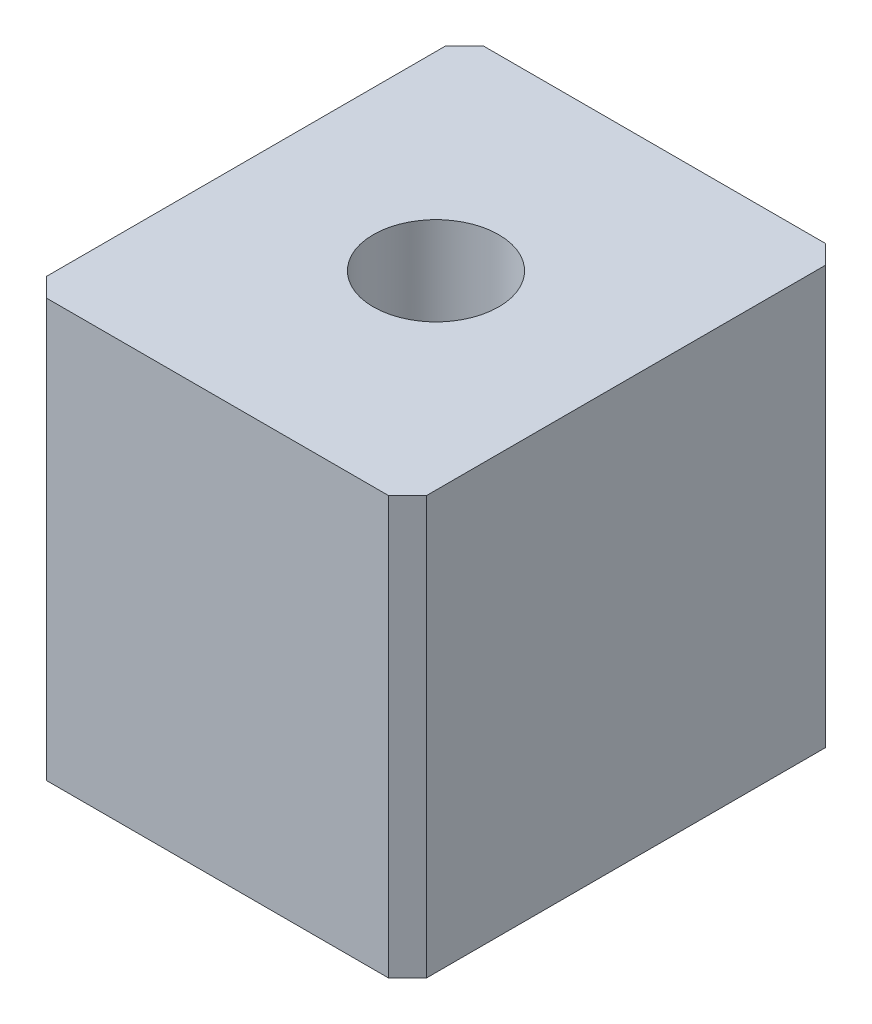
SolidWorks part; units mm, degrees
ref_plane "前视基准面" through (0, 0, 0) normal (0, 0, 1) x (1, 0, 0)
ref_plane "上视基准面" through (0, 0, 0) normal (0, 1, 0) x (1, 0, 0)
ref_plane "右视基准面" through (0, 0, 0) normal (1, 0, 0) x (0, 0, -1)
sketch "草图1" plane through (0, 0, 0) normal (0, 1, 0) x (1, 0, 0)
  line L1 (-10, 11.5) -> (10, 11.5)
  line L2 (-10, 11.5) -> (-10, -11.5)
  line L3 (-10, -11.5) -> (10, -11.5)
  line L4 (10, 11.5) -> (10, -11.5)
  line L5 (-10, 11.5) -> (10, -11.5) construction
  line L6 (-10, -11.5) -> (10, 11.5) construction
  point P0 (0, 0)
  dimension "D1" = 20
  dimension "D2" = 23
extrude "凸台-拉伸1" add sketch "草图1" along normal blind 22
hole_wizard "M6 六角凹头螺钉的柱形沉头孔1" positions "草图5" profile "草图4" counterbore size "M6" standard "ISO"
sketch "草图5" plane through (0, 0, 0) normal (0, -1, 0) x (-1, 0, 0)
  point P0 (0, 0)
sketch "草图4" plane through (0, 0, 0) normal (1, 0, 0) x (0, 0, -1)
  line L0 (0, 0) -> (0, 24.2328)
  line L1 (0, 24.2328) -> (3.3, 22.25)
  line L2 (3.3, 22.25) -> (3.3, 15)
  line L3 (3.3, 15) -> (5.5, 15)
  line L4 (5.5, 15) -> (5.5, 0)
  line L5 (5.5, 0) -> (0, 0)
  line L10 (0, 24.2328) -> (-3.3, 22.25) construction
  line L11 (0, -6.35) -> (0, 107.95) construction
  dimension "孔直径" = 6.6
  dimension "孔深度" = 22.25
  dimension "柱形沉头孔直径" = 11
  dimension "柱形沉头孔深度" = 15
  dimension "导头角度" = 118
chamfer "倒角1" distance 1 angle 45 4 edges at (10, 11, 11.5) (10, 11, -11.5) (-10, 11, -11.5) (-10, 11, 11.5)
